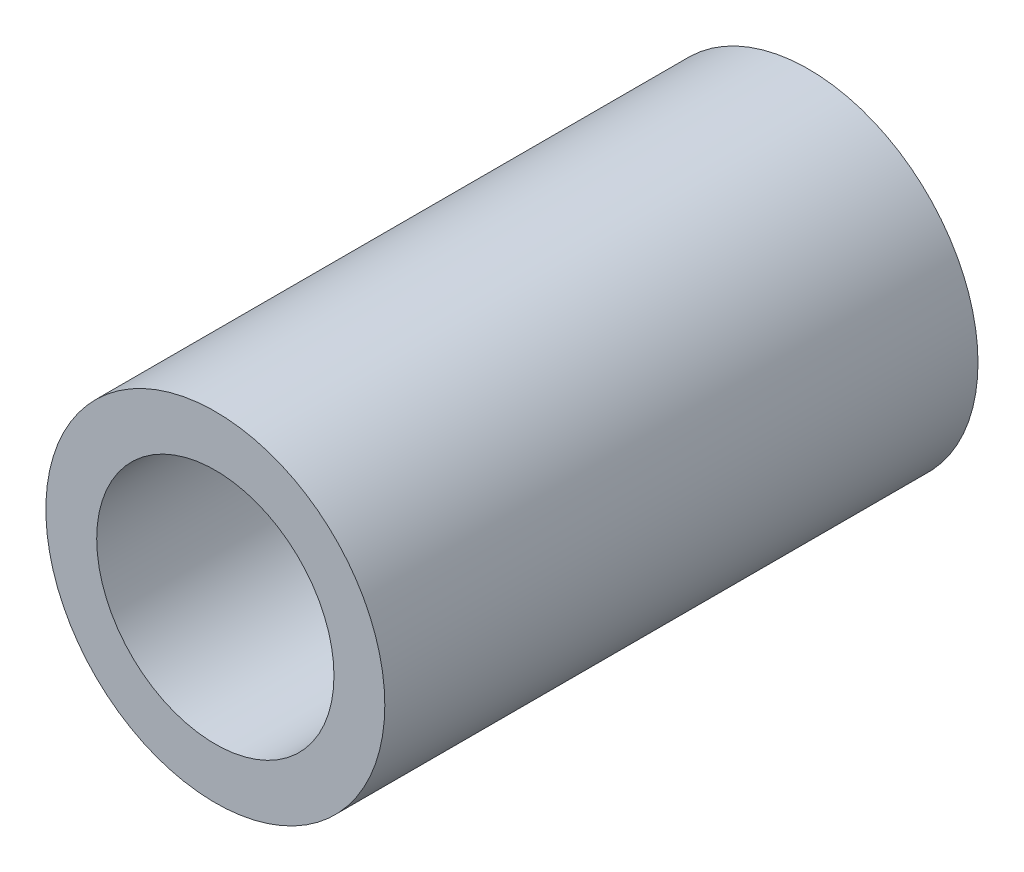
SolidWorks part; units mm, degrees
material "Q235B"
ref_plane "Front Plane" through (0, 0, 0) normal (0, 0, 1) x (1, 0, 0)
ref_plane "Top Plane" through (0, 0, 0) normal (0, 1, 0) x (1, 0, 0)
ref_plane "Right Plane" through (0, 0, 0) normal (1, 0, 0) x (0, 0, -1)
sketch "Sketch1" plane through (0, 0, 0) normal (0, 0, 1) x (1, 0, 0)
  circle A0 centre (0, 0) radius 10
  circle A1 centre (0, 0) radius 7
  dimension "D1" = 20
  dimension "D2" = 3
extrude "Boss-Extrude1" add sketch "Sketch1" along normal blind 35
